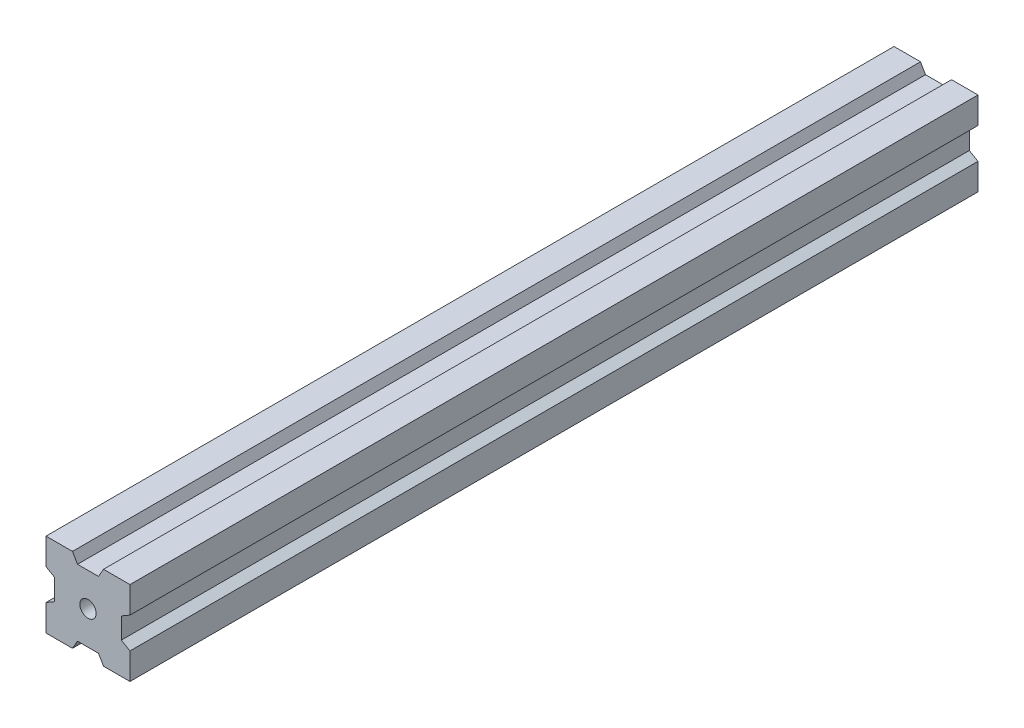
from build123d import *

# Parameters (mm, degrees)
SKETCH_1_W               = 20
SKETCH_1_H               = 20
SKETCH_1_R               = 1.94442565
EXTRUDE_1_DEPTH          = 101
CUT_EXTRUDE_1_DEPTH      = 203.494444368
PATTERN_CIRCULAR_1_COUNT = 4


with BuildPart() as part:
    # 草图1 → 凸台-拉伸1 (new, symmetric)
    with BuildSketch(Plane.XY):
        Rectangle(SKETCH_1_W, SKETCH_1_H)
        Circle(SKETCH_1_R, mode=Mode.SUBTRACT)
    extrude(amount=EXTRUDE_1_DEPTH, both=True)

    # 草图2 → 切除-拉伸1 (cut, symmetric)
    with BuildSketch(Plane.XY.offset(101)):
        Polygon((-32.933615203, 60.643738676), (-3.694439046, 10), (-2.5, 7.931170886), (2.5, 7.931170886), (3.694439046, 10), (32.933615203, 60.643738676), (32.933615203, 177.600443305), (-32.933615203, 177.600443305), align=None)
    cut_extrude_1 = extrude(amount=CUT_EXTRUDE_1_DEPTH, both=True, mode=Mode.SUBTRACT)

    # 阵列(圆周)1: 切除-拉伸1 ×4 about axis
    pattern_circular_1_axis = Axis((0, 0, 101), (0, 0, -1))
    for i in range(1, PATTERN_CIRCULAR_1_COUNT):
        add(cut_extrude_1.rotate(pattern_circular_1_axis, i * 360 / PATTERN_CIRCULAR_1_COUNT), mode=Mode.SUBTRACT)


solid = part.part
